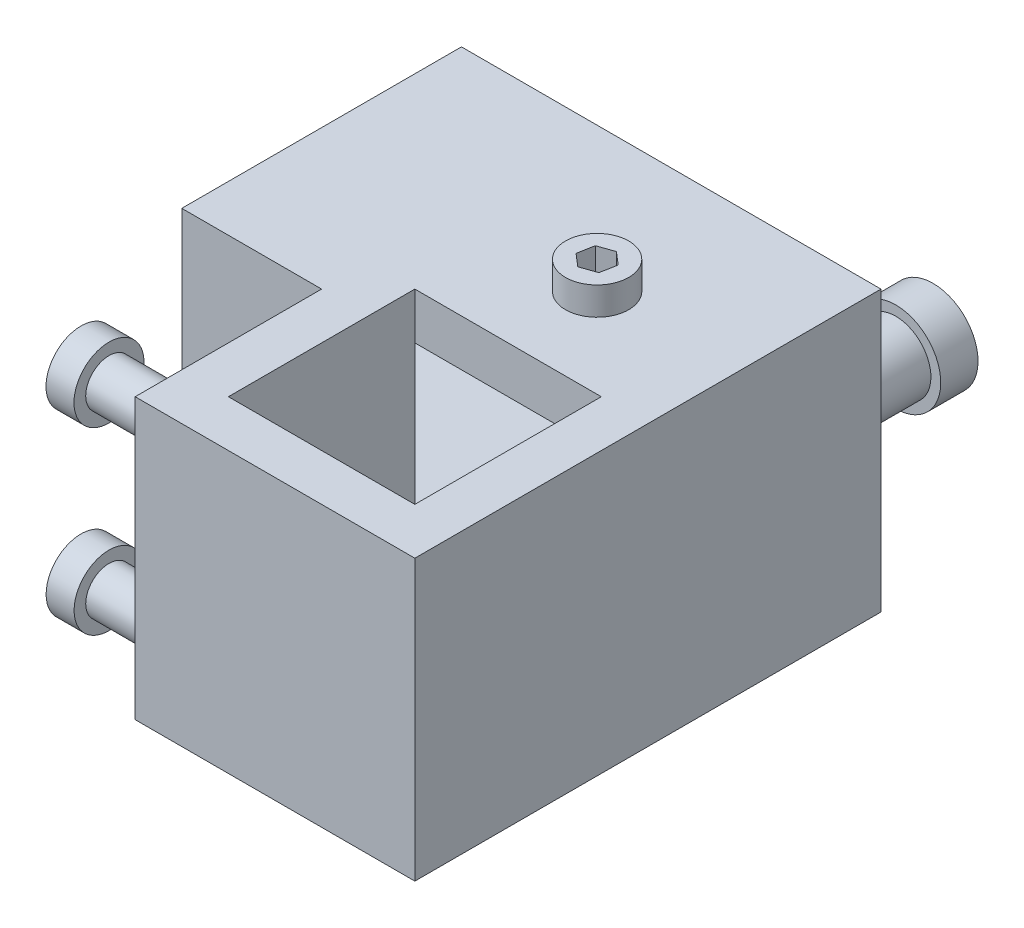
SolidWorks part; units mm, degrees
ref_plane "Front Plane" through (0, 0, 0) normal (0, 0, 1) x (1, 0, 0)
ref_plane "Top Plane" through (0, 0, 0) normal (0, 1, 0) x (1, 0, 0)
ref_plane "Right Plane" through (0, 0, 0) normal (1, 0, 0) x (0, 0, -1)
other "Configuration Table"
sketch "Sketch1" plane through (0, 0, 0) normal (0, 1, 0) x (1, 0, 0)
  line L1 (-30, 30) -> (30, 30)
  line L2 (-30, 30) -> (-30, -30)
  line L3 (-30, -30) -> (30, -30)
  line L4 (30, 30) -> (30, -30)
  line L5 (-30, 30) -> (30, -30) construction
  line L6 (-30, -30) -> (30, 30) construction
  line L7 (-20, 20) -> (20, 20)
  line L8 (-20, 20) -> (-20, -20)
  line L9 (-20, -20) -> (20, -20)
  line L10 (20, 20) -> (20, -20)
  line L11 (-20, 20) -> (20, -20) construction
  line L12 (-20, -20) -> (20, 20) construction
  point P0 (0, 0)
  point P6 (0, 0)
  dimension "D1" = 60
  dimension "D2" = 60
  dimension "D3" = 40
  dimension "D4" = 40
extrude "Boss-Extrude1" add sketch "Sketch1" along normal blind 60
sketch "Sketch2" plane through (-30, 0, 0) normal (-1, 0, 0) x (0, 0, 1)
  line L0 (-30, 0) -> (30, 0) construction
  line L1 (-30, 60) -> (-70, 60)
  line L2 (-30, 60) -> (-30, 0) construction
  line L3 (-30, 0) -> (-70, 0)
  line L4 (-70, 60) -> (-70, 0)
  line L5 (-30, 60) -> (-10, 60)
  line L6 (-30, 60) -> (-30, 0) construction
  line L7 (-30, 0) -> (-10, 0)
  line L8 (-10, 60) -> (-10, 0)
  dimension "D1" = 40
  dimension "D2" = 20
extrude "Boss-Extrude2" add sketch "Sketch2" against normal blind 60 and the other way blind 30
sketch "Sketch3" plane through (-30, 0, 0) normal (-1, 0, 0) x (0, 0, 1)
  line L0 (-10, 60) -> (30, 60) construction
  line L1 (-60, 50) -> (-20, 50)
  line L2 (-60, 50) -> (-60, 10)
  line L3 (-60, 10) -> (-20, 10)
  line L4 (-20, 50) -> (-20, 10)
  line L5 (-70, 60) -> (-70, 0) construction
  dimension "D1" = 10
  dimension "D2" = 40
  dimension "D3" = 40
  dimension "D4" = 10
extrude "Cut-Extrude1" cut sketch "Sketch3" against normal blind 50 and the other way blind 50
sketch "Sketch4" plane through (0, 60, 0) normal (0, 1, 0) x (1, 0, 0)
  line L1 (-20, 10) -> (20, 10)
  line L2 (-20, 10) -> (-20, 20)
  line L3 (-20, 20) -> (20, 20)
  line L4 (20, 10) -> (20, 20)
  dimension "D1" = 40
  dimension "D2" = 10
extrude "Cut-Extrude2" cut sketch "Sketch4" against normal blind 60
sketch "Sketch5" plane through (0, 0, -70) normal (0, 0, -1) x (-1, 0, 0)
  circle A0 centre (-14.1645, 30) radius 9.6508
extrude "Boss-Extrude3" add sketch "Sketch5" along normal blind 4
sketch "Sketch6" plane through (0, 0, -74) normal (0, 0, -1) x (-1, 0, 0)
  circle A0 centre (-14.1645, 30) radius 7.5436
extrude "Boss-Extrude4" add sketch "Sketch6" along normal blind 15
sketch "Sketch7" plane through (0, 0, -89) normal (0, 0, -1) x (-1, 0, 0)
  circle A0 centre (-14.1645, 30) radius 9.6508
extrude "Boss-Extrude5" add sketch "Sketch7" along normal blind 8
sketch "Sketch8" plane through (0, 0, -70) normal (0, 0, -1) x (-1, 0, 0)
  circle A0 centre (13.7828, 47) radius 3
  circle A1 centre (13.7828, 13) radius 3
  circle A2 centre (-14.1645, 30) radius 9.6508 construction
  dimension "D1" = 17
  dimension "D2" = 17
  dimension "D3" = 6
  dimension "D4" = 6
extrude "Cut-Extrude3" cut sketch "Sketch8" against normal blind 18
sketch "Sketch9" plane through (0, 0, -70) normal (0, 0, -1) x (-1, 0, 0)
  line L1 (47.5727, 45.7264) -> (48.1073, 47.7217)
  line L2 (48.1073, 47.7217) -> (46.6467, 49.1824)
  line L3 (46.6467, 49.1824) -> (44.6514, 48.6477)
  line L4 (44.6514, 48.6477) -> (44.1167, 46.6524)
  line L5 (44.1167, 46.6524) -> (45.5774, 45.1918)
  line L6 (45.5774, 45.1918) -> (47.5727, 45.7264)
  line L7 (47.5727, 11.3523) -> (47.8543, 13.2015)
  line L8 (47.8543, 13.2015) -> (46.3937, 14.37)
  line L9 (46.3937, 14.37) -> (44.6514, 13.6893)
  line L10 (44.6514, 13.6893) -> (44.3697, 11.8401)
  line L11 (44.3697, 11.8401) -> (45.8304, 10.6716)
  line L12 (45.8304, 10.6716) -> (47.5727, 11.3523)
  circle A0 centre (46.112, 47.1871) radius 3.7271
  circle A1 centre (46.112, 12.5208) radius 3.6811
  circle A2 centre (46.112, 47.1871) radius 1.7889 construction
  circle A3 centre (46.112, 12.5208) radius 1.6199 construction
extrude "Boss-Extrude6" add sketch "Sketch9" along normal blind 4
sketch "Sketch10" plane through (0, 60, 0) normal (0, 1, 0) x (1, 0, 0)
  line L1 (2.6936, 36.7898) -> (3.3488, 40.2783)
  line L2 (3.3488, 40.2783) -> (0.6552, 42.59)
  line L3 (0.6552, 42.59) -> (-2.6936, 41.4132)
  line L4 (-2.6936, 41.4132) -> (-3.3488, 37.9246)
  line L5 (-3.3488, 37.9246) -> (-0.6552, 35.6129)
  line L6 (-0.6552, 35.6129) -> (2.6936, 36.7898)
  circle A0 centre (0, 39.1015) radius 6.7811
  circle A1 centre (0, 39.1015) radius 3.074 construction
extrude "Boss-Extrude7" add sketch "Sketch10" along normal blind 6
sketch "Sketch11" plane through (0, 0, 0) normal (0, -1, 0) x (1, 0, 0)
  line L1 (2.3379, -39.9906) -> (3.633, -36.5433)
  line L2 (3.633, -36.5433) -> (1.2951, -33.6981)
  line L3 (1.2951, -33.6981) -> (-2.3379, -34.3002)
  line L4 (-2.3379, -34.3002) -> (-3.633, -37.7475)
  line L5 (-3.633, -37.7475) -> (-1.2951, -40.5927)
  line L6 (-1.2951, -40.5927) -> (2.3379, -39.9906)
  circle A0 centre (0, -37.1454) radius 6.5417
  circle A1 centre (0, -37.1454) radius 3.1892 construction
extrude "Boss-Extrude8" add sketch "Sketch11" along normal blind 6
sketch "Sketch12" plane through (-30, 0, 0) normal (-1, 0, 0) x (0, 0, 1)
  circle A0 centre (19.609, 49.4435) radius 5
  circle A1 centre (19.609, 10.8313) radius 5
  dimension "D1" = 10
  dimension "D2" = 10
extrude "Boss-Extrude9" add sketch "Sketch12" along normal blind 16
sketch "Sketch13" plane through (-46, 0, 0) normal (-1, 0, 0) x (0, 0, 1)
  line L1 (22.8097, 46.8485) -> (23.4567, 50.9179)
  line L2 (23.4567, 50.9179) -> (20.256, 53.513)
  line L3 (20.256, 53.513) -> (16.4083, 52.0386)
  line L4 (16.4083, 52.0386) -> (15.7613, 47.9691)
  line L5 (15.7613, 47.9691) -> (18.962, 45.3741)
  line L6 (18.962, 45.3741) -> (22.8097, 46.8485)
  line L7 (22.2463, 7.0241) -> (24.2248, 11.2117)
  line L8 (24.2248, 11.2117) -> (21.5875, 15.0189)
  line L9 (21.5875, 15.0189) -> (16.9717, 14.6385)
  line L10 (16.9717, 14.6385) -> (14.9932, 10.4509)
  line L11 (14.9932, 10.4509) -> (17.6305, 6.6437)
  line L12 (17.6305, 6.6437) -> (22.2463, 7.0241)
  circle A0 centre (19.609, 10.8313) radius 7.492
  circle A1 centre (19.609, 49.4435) radius 7.5174
  circle A2 centre (19.609, 49.4435) radius 3.5685 construction
  circle A3 centre (19.609, 10.8313) radius 4.0109 construction
extrude "Boss-Extrude10" add sketch "Sketch13" along normal blind 6
